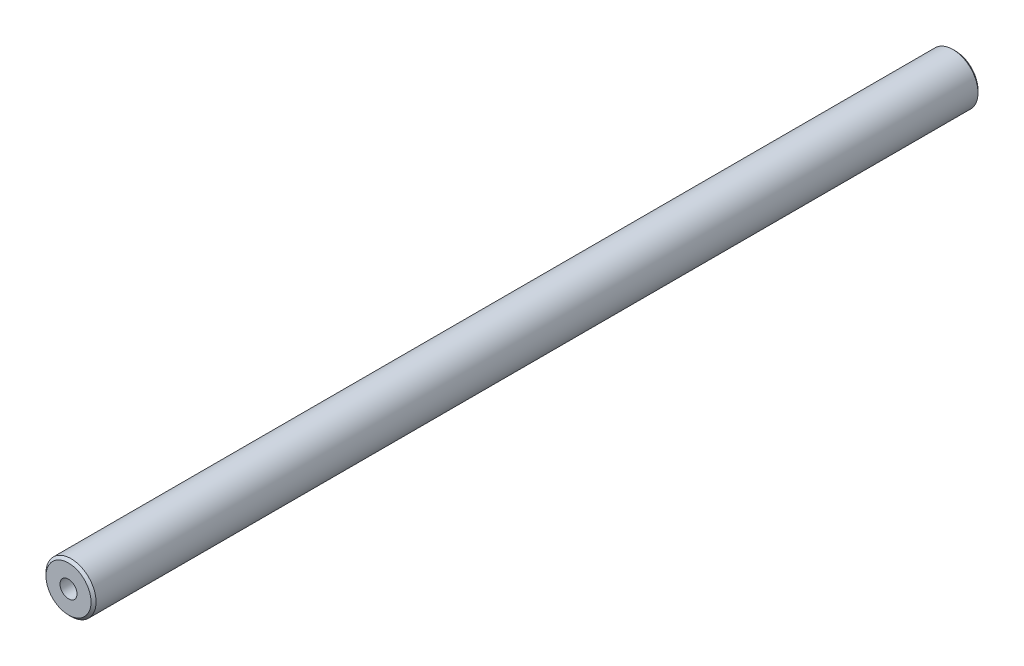
from build123d import *

# Parameters (mm, degrees)
SKETCH_1_R             = 10
EXTRUDE_1_DEPTH        = 177
HOLE_WIZARD_M8_1_D     = 6.8
HOLE_WIZARD_M8_1_DEPTH = 19.75
HOLE_WIZARD_M8_1_TIP   = 2.042926105
HOLE_WIZARD_M8_2_D     = 6.8
HOLE_WIZARD_M8_2_DEPTH = 19.75
HOLE_WIZARD_M8_2_TIP   = 2.042926105
CHAMFER_1_SIZE         = 1


with BuildPart() as part:
    # 草图1 → 凸台-拉伸1 (new, symmetric)
    with BuildSketch(Plane.XY):
        Circle(SKETCH_1_R)
    extrude(amount=EXTRUDE_1_DEPTH, both=True)

    # M8 螺纹孔1
    with Locations(Plane(origin=(0, 0, -177), x_dir=(-1, 0, 0), z_dir=(0, 0, -1))):
        with Locations((0, 0)):
            Hole(HOLE_WIZARD_M8_1_D / 2, depth=HOLE_WIZARD_M8_1_DEPTH)
            with Locations((0, 0, -(HOLE_WIZARD_M8_1_DEPTH + HOLE_WIZARD_M8_1_TIP / 2))):  # 118° drill point
                Cone(0, HOLE_WIZARD_M8_1_D / 2, HOLE_WIZARD_M8_1_TIP, mode=Mode.SUBTRACT)

    # M8 螺纹孔2
    with Locations(Plane.XY.offset(177)):
        with Locations((0, 0)):
            Hole(HOLE_WIZARD_M8_2_D / 2, depth=HOLE_WIZARD_M8_2_DEPTH)
            with Locations((0, 0, -(HOLE_WIZARD_M8_2_DEPTH + HOLE_WIZARD_M8_2_TIP / 2))):  # 118° drill point
                Cone(0, HOLE_WIZARD_M8_2_D / 2, HOLE_WIZARD_M8_2_TIP, mode=Mode.SUBTRACT)

    # 倒角1
    chamfer_1_edges = [part.edges().sort_by_distance(p)[0] for p in [
        (-10, 0, -177),
        (-10, 0, 177),
    ]]
    chamfer(chamfer_1_edges, length=CHAMFER_1_SIZE)


solid = part.part
